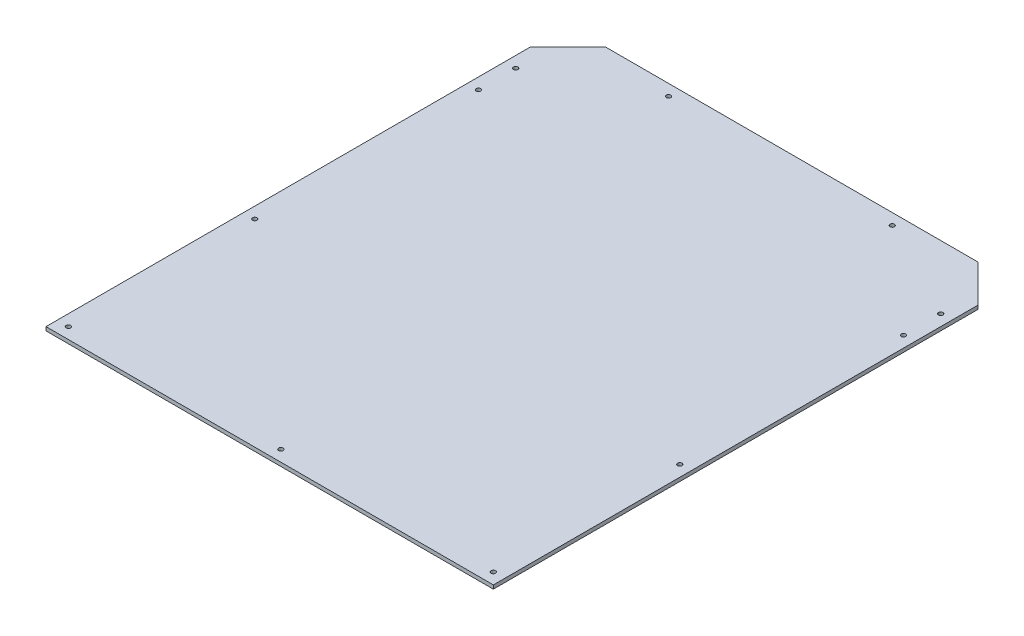
SolidWorks part; units mm, degrees
ref_plane "前视" through (0, 0, 0) normal (0, 0, 1) x (1, 0, 0)
ref_plane "上视" through (0, 0, 0) normal (0, 1, 0) x (1, 0, 0)
ref_plane "右视" through (0, 0, 0) normal (1, 0, 0) x (0, 0, -1)
sketch "草图1" plane through (0, 0, 0) normal (0, 1, 0) x (1, 0, 0)
  line L0 (0, 650) -> (50, 700)
  line L1 (0, 0) -> (600, 0)
  line L2 (0, 0) -> (0, 650)
  line L3 (50, 700) -> (550, 700)
  line L4 (600, 0) -> (600, 650)
  line L5 (550, 700) -> (600, 650)
  point P1 (600, 700)
  point P2 (0, 700)
  dimension "D1" = 700
  dimension "D2" = 600
extrude "凸台-拉伸1" add sketch "草图1" along normal blind 5
sketch "草图2" plane through (0, 5, 0) normal (0, 1, 0) x (1, 0, 0)
  line L0 (15, 15) -> (15, 823.1709) construction
  line L1 (0, 650) -> (0, 0) construction
  line L2 (0, 0) -> (600, 0) construction
  line L3 (550, 700) -> (50, 700) construction
  line L4 (300, 0) -> (300, 823.1709) construction
  circle A0 centre (15, 15) radius 3
  circle A1 centre (15, 265) radius 3
  circle A2 centre (15, 565) radius 3
  circle A3 centre (15, 615) radius 3
  circle A4 centre (150, 685) radius 3
  circle A5 centre (585, 15) radius 3
  circle A6 centre (585, 265) radius 3
  circle A7 centre (585, 565) radius 3
  circle A8 centre (585, 615) radius 3
  circle A9 centre (450, 685) radius 3
  circle A10 centre (300, 15) radius 3
  dimension "D2" = 6
  dimension "D3" = 6
  dimension "D4" = 6
  dimension "D5" = 15
  dimension "D6" = 250
  dimension "D7" = 6
  dimension "D8" = 300
  dimension "D9" = 50
  dimension "D10" = 6
  dimension "D11" = 15
  dimension "D12" = 100
  dimension "D13" = 6
  dimension "D14" = 15
  dimension "D1" = 15
extrude "切除-拉伸1" cut sketch "草图2" against normal blind 10
